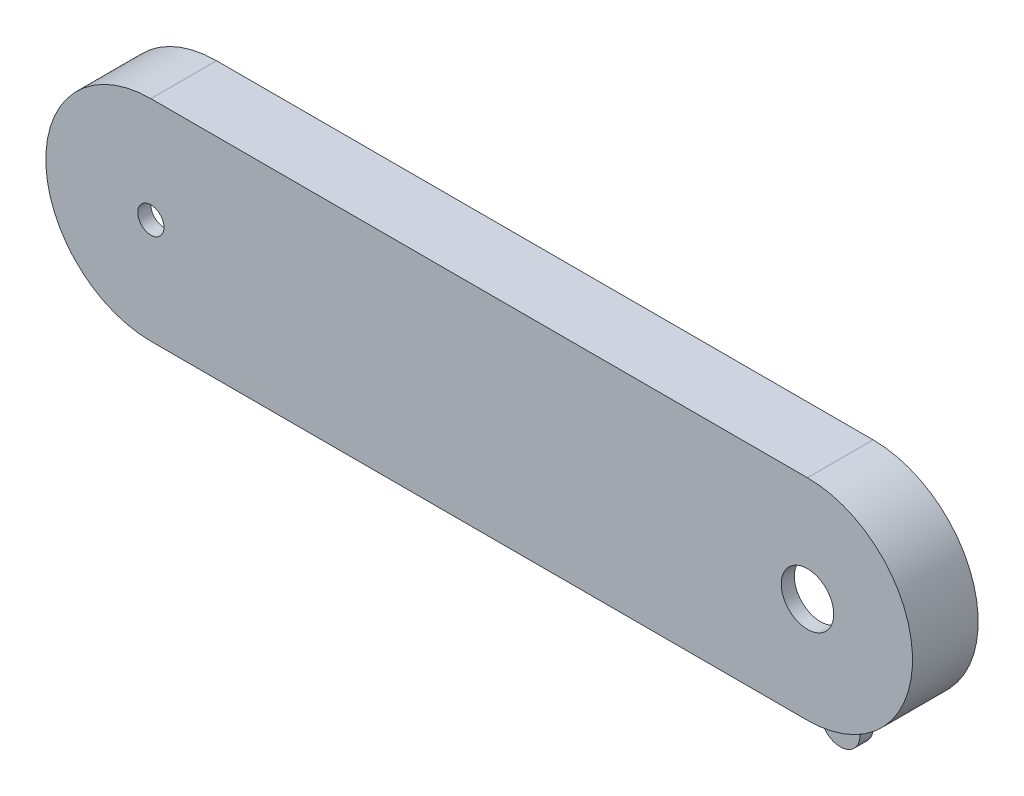
from build123d import *

# Parameters (mm, degrees)
SKETCH_1_R      = 20
SKETCH_1_R_2    = 10
EXTRUDE_1_DEPTH = 10
EXTRUDE_START   = 40
EXTRUDE_2_DEPTH = 40
SKETCH_4_R      = 5
EXTRUDE_3_DEPTH = 10


with BuildPart() as part:
    # 草图1 → 凸台-拉伸1 (new body)
    with BuildSketch(Plane.XY):
        with BuildLine():
            Line((0, 80), (-500, 80))
            ThreePointArc((-500, 80), (-580, 0), (-500, -80))
            Line((-500, -80), (0, -80))
            ThreePointArc((0, -80), (80, 0), (0, 80))
        make_face()
        Circle(SKETCH_1_R, mode=Mode.SUBTRACT)
        with Locations((-500, 0)):
            Circle(SKETCH_1_R_2, mode=Mode.SUBTRACT)
    extrude(amount=EXTRUDE_1_DEPTH)

    # 草图2 → 凸台-拉伸2 (add)
    with BuildSketch(Plane(origin=(0, 0, 0), x_dir=(-1, 0, 0), z_dir=(0, 0, -1)).offset(EXTRUDE_START)):
        with BuildLine():
            Line((0, -80), (500, -80))
            ThreePointArc((500, -80), (580, 0), (500, 80))
            Line((500, 80), (0, 80))
            ThreePointArc((0, 80), (-80, 0), (0, -80))
        make_face()
        with BuildLine():
            Line((0, -70), (500, -70))
            ThreePointArc((500, -70), (570, 0), (500, 70))
            Line((500, 70), (0, 70))
            ThreePointArc((0, 70), (-70, 0), (0, -70))
        make_face(mode=Mode.SUBTRACT)
    extrude(amount=-EXTRUDE_2_DEPTH)

    # 草图4 → 凸台-拉伸3 (add)
    with BuildSketch(Plane(origin=(0, 0, -40), x_dir=(-1, 0, 0), z_dir=(0, 0, -1))):
        with BuildLine():
            Line((30, -110), (30, -80))
            Line((30, -80), (0, -80))
            Line((0, -80), (0, -110))
            ThreePointArc((0, -110), (15, -125.000001141), (30, -110))
        make_face()
        with Locations(Location((15, -110.000001141, 0), (0, 0, 180))):
            Circle(SKETCH_4_R, mode=Mode.SUBTRACT)
    extrude(amount=-EXTRUDE_3_DEPTH)


solid = part.part
